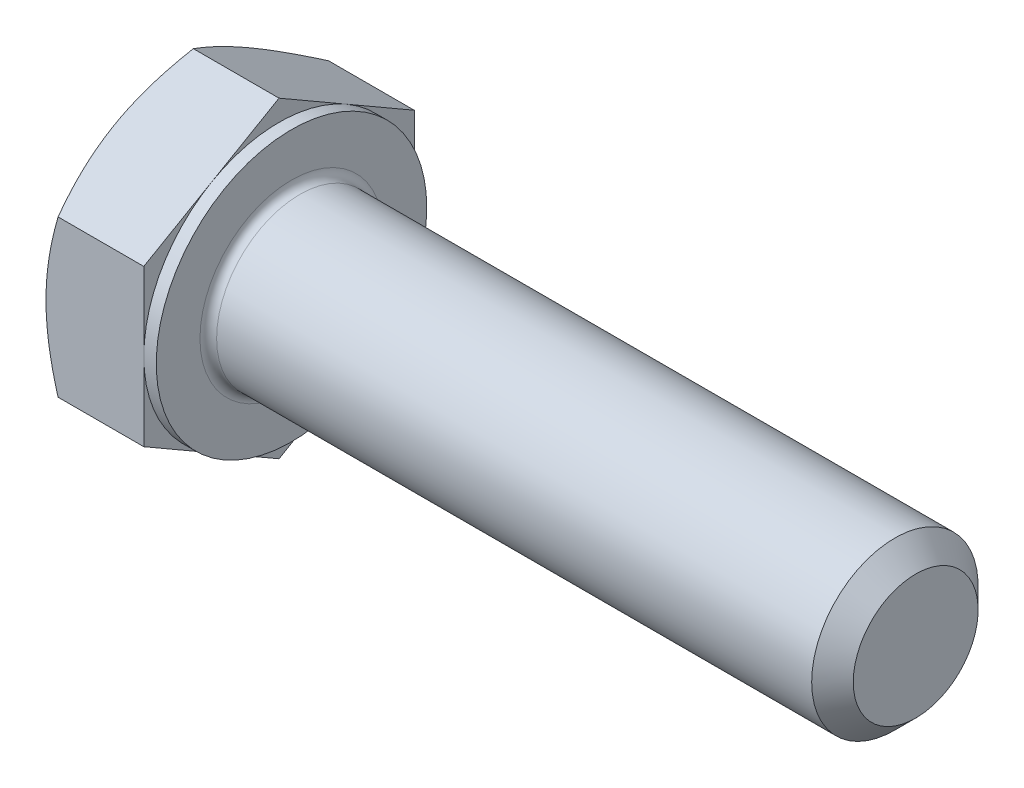
from build123d import *

# Parameters (mm, degrees)
EXTRUDE_368_DEPTH = 5.3
SKETCH_4_W        = 0.6
SKETCH_4_H        = 11.005553499
CHAMFER_1891_SIZE = 1
FILLET_1936_R     = 0.4


with BuildPart() as part:
    # 草图1 → Extrude 368 (new body)
    with BuildSketch(Plane(origin=(0, 0, 0), x_dir=(0, 0, -1), z_dir=(1, 0, 0))):
        Polygon((6.5, 3.75277675), (6.5, -3.75277675), (0, -7.505553499), (-6.5, -3.75277675), (-6.5, 3.75277675), (0, 7.505553499), align=None)
    extrude(amount=EXTRUDE_368_DEPTH)

    # 草图2 → 凸台-旋转1 (revolve)
    with BuildSketch(Plane.XY, mode=Mode.PRIVATE) as revolve_1_sk:
        Polygon((0, 0), (35.3, 0), (35.3, 2.9175), (35.3, 4), (0, 4), align=None)
    revolve(revolve_1_sk.sketch.rotate(Axis((0, 0, 0), (1, 0, 0)), 90), axis=Axis((0, 0, 0), (1, 0, 0)))

    # 草图3 → 切除-旋转1 (revolve, cut)
    with BuildSketch(Plane.XY):
        Polygon((0, 6.5), (3.46730793, 12.505553499), (3.46730793, 17.505553499), (-10, 17.505553499), (-10, 6.5), align=None)
    revolve(axis=Axis((0, 0, 0), (1, 0, 0)), mode=Mode.SUBTRACT)

    # 草图5 → 切除-旋转2 (revolve, cut)
    with BuildSketch(Plane.XY):
        Polygon((5.3, 6.5), (1.83269207, 12.505553499), (1.83269207, 17.505553499), (11.83269207, 17.505553499), (11.83269207, 6.5), align=None)
    revolve(axis=Axis((0, 0, 0), (1, 0, 0)), mode=Mode.SUBTRACT)

    # 草图4 → 切除-旋转3 (revolve, cut)
    with BuildSketch(Plane.XY, mode=Mode.PRIVATE) as cut_revolve_3_sk:
        with Locations((5, 12.00277675)):
            Rectangle(SKETCH_4_W, SKETCH_4_H)
    revolve(cut_revolve_3_sk.sketch.rotate(Axis((0, 0, 0), (1, 0, 0)), 270), axis=Axis((0, 0, 0), (1, 0, 0)), mode=Mode.SUBTRACT)

    # Chamfer 1891
    chamfer_1891_edges = [part.edges().sort_by_distance(p)[0] for p in [
        (35.3, 0, -4),
    ]]
    chamfer(chamfer_1891_edges, length=CHAMFER_1891_SIZE)

    # Fillet 1936
    fillet_1936_edges = [part.edges().sort_by_distance(p)[0] for p in [
        (5.3, 0, -4),
    ]]
    fillet(fillet_1936_edges, radius=FILLET_1936_R)


solid = part.part
